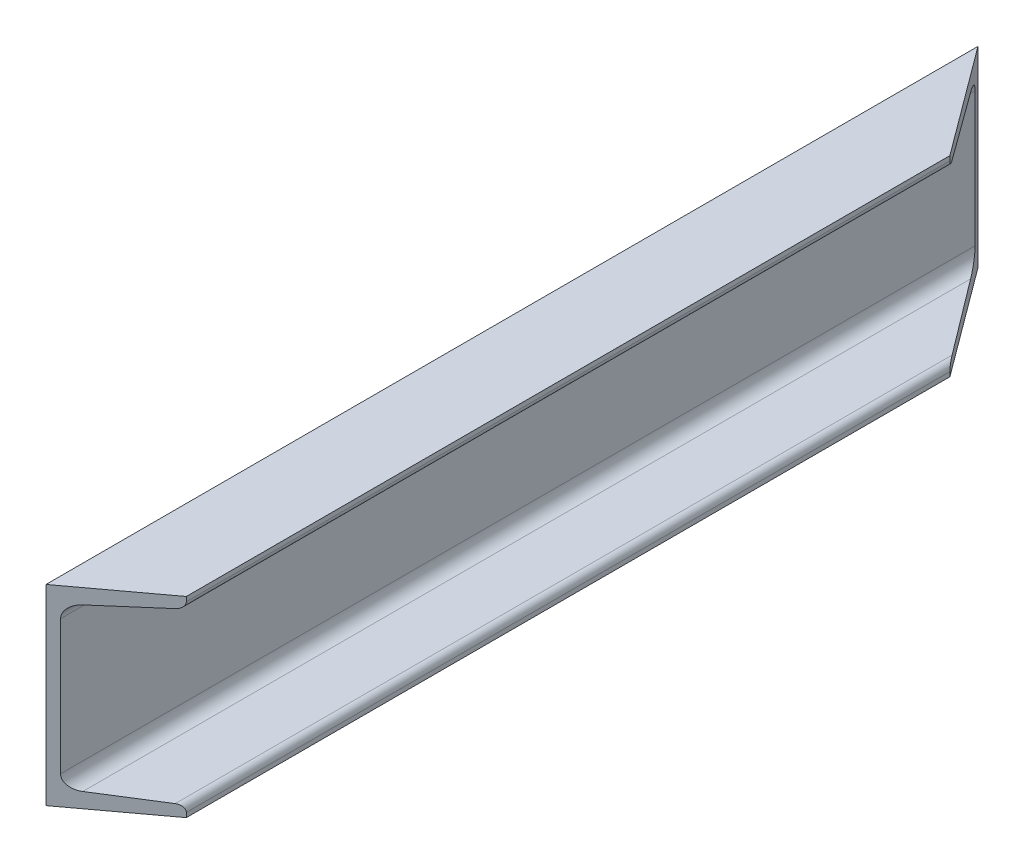
from build123d import *

# Parameters (mm, degrees)
BOSS_EXTRUDE1_DEPTH = 306.5
CUT_EXTRUDE1_DEPTH  = 613


with BuildPart() as part:
    # Sketch1 → Boss-Extrude1 (new, symmetric)
    with BuildSketch(Plane.XY):
        with BuildLine():
            Line((0, 63), (0, -63))
            Line((0, -63), (53, -63))
            Line((53, -63), (53, -60.015930389))
            ThreePointArc((53, -60.015930389), (51.788680261, -56.944353898), (48.806852383, -55.526404621))
            Line((48.806852383, -55.526404621), (13.886295235, -53.139636681))
            ThreePointArc((13.886295235, -53.139636681), (7.922639477, -50.303738128), (5.5, -44.160585147))
            Line((5.5, -44.160585147), (5.5, 44.160585147))
            ThreePointArc((5.5, 44.160585147), (7.922639477, 50.303738128), (13.886295235, 53.139636681))
            Line((13.886295235, 53.139636681), (48.806852383, 55.526404621))
            ThreePointArc((48.806852383, 55.526404621), (51.788680261, 56.944353898), (53, 60.015930389))
            Line((53, 60.015930389), (53, 63))
            Line((53, 63), (0, 63))
        make_face()
    extrude(amount=BOSS_EXTRUDE1_DEPTH, both=True)

    # Sketch2 → Cut-Extrude1 (cut)
    with BuildSketch(Plane(origin=(0, 63, 0), x_dir=(1, 0, 0), z_dir=(0, 1, 0))):
        Polygon((0, -306.5), (53, -267.210441025), (53, -306.5), align=None)
        Polygon((0, 306.5), (53, 235.005178647), (53, 306.5), align=None)
    extrude(amount=-CUT_EXTRUDE1_DEPTH, mode=Mode.SUBTRACT)


solid = part.part
